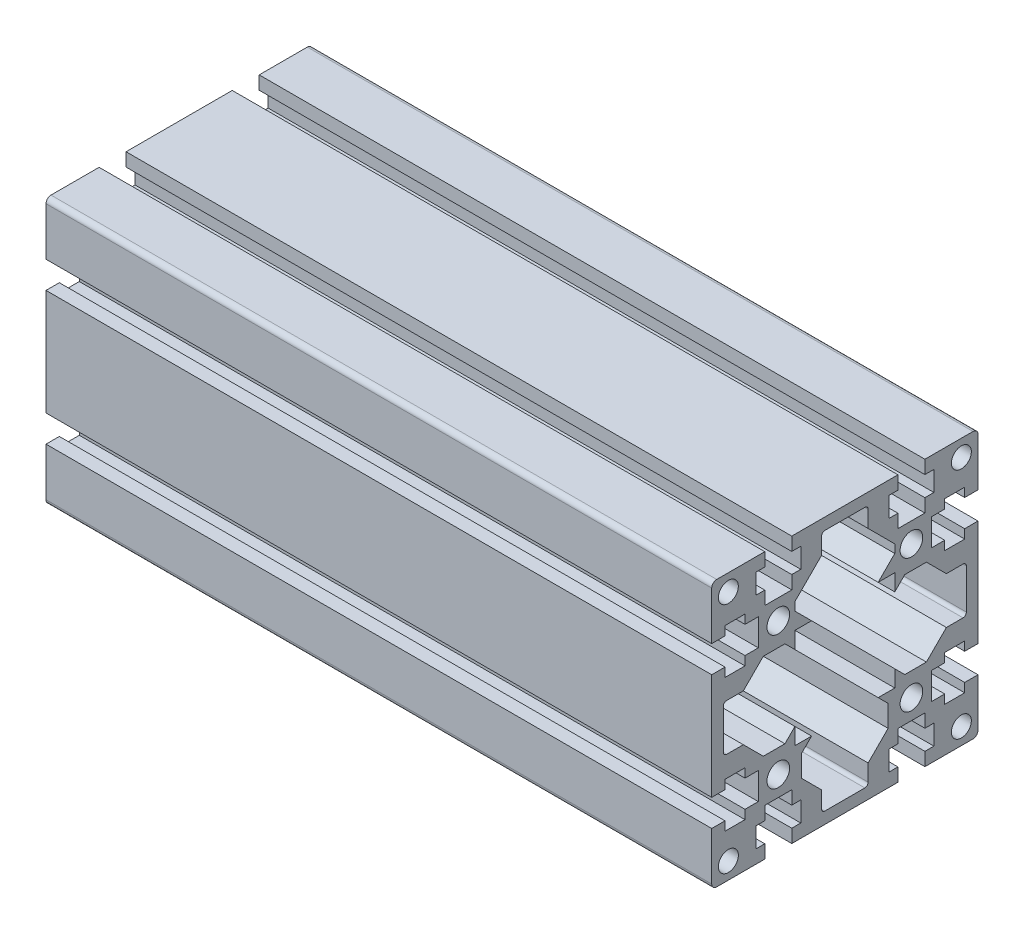
SolidWorks part; units mm, degrees
ref_plane "Front Plane" through (0, 0, 0) normal (0, 0, 1) x (1, 0, 0)
ref_plane "Top Plane" through (0, 0, 0) normal (0, 1, 0) x (1, 0, 0)
ref_plane "Right Plane" through (0, 0, 0) normal (1, 0, 0) x (0, 0, -1)
sketch "草图1" plane through (0, 0, 0) normal (0, 0, 1) x (1, 0, 0)
  line L0 (-530.3448, 0) -> (-330.3448, 0)
  dimension "D1" = 200
other "Aluminium profile 80 X 80G X R1.5(1)"
ref_plane "Plane2" through (-530.3448, 0, 0) normal (1, 0, 0) x (0, 1, 0)
sketch "Sketch1" plane through (-530.3448, 0, 0) normal (1, 0, 0) x (0, 1, 0)
  line L0 (0, 40) -> (0, 0) construction
  line L1 (0, 0) -> (40, 0) construction
  line L2 (-24.05, 40) -> (-24.05, 36)
  line L3 (-38.5, 40) -> (-24.05, 40)
  line L4 (-40, 38.5) -> (-40, 24.05)
  line L5 (-38.5, -40) -> (-24.05, -40)
  line L6 (40, 38.5) -> (40, 24.05)
  line L7 (-24.05, 36) -> (-26.75, 36)
  line L8 (-26.75, 36) -> (-26.75, 30)
  line L9 (-26.75, 30) -> (-24.05, 30)
  line L10 (-24.05, 30) -> (-24.05, 26)
  line L11 (-24.05, 26) -> (-15.95, 26)
  line L12 (-15.95, 26) -> (-15.95, 30)
  line L13 (-15.95, 30) -> (-13.25, 30)
  line L14 (-13.25, 30) -> (-13.25, 36)
  line L15 (-13.25, 36) -> (-15.95, 36)
  line L16 (-15.95, 36) -> (-15.95, 40)
  line L17 (-40, 15.95) -> (-36, 15.95)
  line L18 (-36, 15.95) -> (-36, 13.25)
  line L19 (-15.95, 40) -> (15.95, 40)
  line L20 (-20, 20) -> (-20, 40) construction
  line L21 (20, 20) -> (20, 40) construction
  line L22 (15.95, 36) -> (15.95, 40)
  line L23 (13.25, 36) -> (15.95, 36)
  line L24 (13.25, 30) -> (13.25, 36)
  line L25 (15.95, 30) -> (13.25, 30)
  line L26 (-36, 13.25) -> (-30, 13.25)
  line L27 (-30, 13.25) -> (-30, 15.95)
  line L28 (-26, 15.95) -> (-26, 24.05)
  line L29 (-26, 24.05) -> (-30, 24.05)
  line L30 (-30, 24.05) -> (-30, 26.75)
  line L31 (-30, 26.75) -> (-36, 26.75)
  line L32 (-36, 26.75) -> (-36, 24.05)
  line L33 (-36, 24.05) -> (-40, 24.05)
  line L34 (-30, 15.95) -> (-26, 15.95)
  line L35 (15.95, 26) -> (15.95, 30)
  line L36 (24.05, 26) -> (15.95, 26)
  line L37 (24.05, 30) -> (24.05, 26)
  line L38 (26.75, 30) -> (24.05, 30)
  line L39 (26.75, 36) -> (26.75, 30)
  line L40 (24.05, 36) -> (26.75, 36)
  line L41 (24.05, 40) -> (24.05, 36)
  line L42 (24.05, -40) -> (24.05, -36)
  line L43 (24.05, -36) -> (26.75, -36)
  line L44 (26.75, -36) -> (26.75, -30)
  line L45 (26.75, -30) -> (24.05, -30)
  line L46 (24.05, -30) -> (24.05, -26)
  line L47 (24.05, -26) -> (15.95, -26)
  line L48 (15.95, -26) -> (15.95, -30)
  line L49 (15.95, -30) -> (13.25, -30)
  line L50 (13.25, -30) -> (13.25, -36)
  line L51 (13.25, -36) -> (15.95, -36)
  line L52 (15.95, -36) -> (15.95, -40)
  line L53 (-15.95, -36) -> (-15.95, -40)
  line L54 (-13.25, -36) -> (-15.95, -36)
  line L55 (-13.25, -30) -> (-13.25, -36)
  line L56 (-15.95, -30) -> (-13.25, -30)
  line L57 (-15.95, -26) -> (-15.95, -30)
  line L58 (-24.05, -26) -> (-15.95, -26)
  line L59 (-24.05, -30) -> (-24.05, -26)
  line L60 (-26.75, -30) -> (-24.05, -30)
  line L61 (-26.75, -36) -> (-26.75, -30)
  line L62 (-24.05, -36) -> (-26.75, -36)
  line L63 (-24.05, -40) -> (-24.05, -36)
  line L64 (-30, -15.95) -> (-26, -15.95)
  line L65 (-36, -26.75) -> (-36, -24.05)
  line L66 (-30, -26.75) -> (-36, -26.75)
  line L67 (-30, -24.05) -> (-30, -26.75)
  line L68 (-26, -24.05) -> (-30, -24.05)
  line L69 (-26, -15.95) -> (-26, -24.05)
  line L70 (-30, -13.25) -> (-30, -15.95)
  line L71 (-36, -13.25) -> (-30, -13.25)
  line L72 (-36, -15.95) -> (-36, -13.25)
  line L73 (36, 24.05) -> (40, 24.05)
  line L74 (40, 15.95) -> (36, 15.95)
  line L75 (36, -15.95) -> (36, -13.25)
  line L76 (36, -13.25) -> (30, -13.25)
  line L77 (30, -13.25) -> (30, -15.95)
  line L78 (26, -15.95) -> (26, -24.05)
  line L79 (26, -24.05) -> (30, -24.05)
  line L80 (30, -24.05) -> (30, -26.75)
  line L81 (30, -26.75) -> (36, -26.75)
  line L82 (36, -26.75) -> (36, -24.05)
  line L83 (30, -15.95) -> (26, -15.95)
  line L84 (30, 15.95) -> (26, 15.95)
  line L85 (36, 26.75) -> (36, 24.05)
  line L86 (30, 26.75) -> (36, 26.75)
  line L87 (30, 24.05) -> (30, 26.75)
  line L88 (26, 24.05) -> (30, 24.05)
  line L89 (26, 15.95) -> (26, 24.05)
  line L90 (30, 13.25) -> (30, 15.95)
  line L91 (36, 13.25) -> (30, 13.25)
  line L92 (36, 15.95) -> (36, 13.25)
  line L93 (-36, -15.95) -> (-40, -15.95)
  line L94 (-36, -24.05) -> (-40, -24.05)
  line L95 (36, -15.95) -> (40, -15.95)
  line L96 (36, -24.05) -> (40, -24.05)
  line L97 (-13, 18) -> (-10, 15)
  line L98 (-15, 15) -> (-10, 15)
  line L99 (-15, 15) -> (-15, 10)
  line L100 (-15, -15) -> (-10, -15)
  line L101 (15, 15) -> (15, 10)
  line L102 (-18, 13) -> (-15, 10)
  line L104 (13, 18) -> (10, 15)
  line L105 (13, -18) -> (10, -15)
  line L106 (20, -15) -> (15, -10)
  line L107 (-18, -13) -> (-15, -10)
  line L108 (-13, -18) -> (-10, -15)
  line L109 (15, -10) -> (15, -15)
  line L110 (10, 15) -> (15, 15)
  line L111 (-15, -10) -> (-15, -15)
  line L112 (10, -15) -> (15, -15)
  line L113 (15, 10) -> (20, 15)
  line L235 (24.05, 40) -> (38.5, 40)
  line L249 (-40, 15.95) -> (-40, -15.95)
  line L250 (-20, 20) -> (-26, 20) construction
  line L264 (40, 15.95) -> (40, -15.95)
  line L265 (-13, 24.5) -> (-7, 30.5)
  line L266 (-7, 30.5) -> (-7, 35.5)
  line L267 (7, 35.5) -> (7, 30.5)
  line L268 (7, 30.5) -> (13, 24.5)
  line L269 (-6, -36.5) -> (6, -36.5)
  line L270 (-13, 24.5) -> (-13, 18)
  line L271 (-35.5, 7) -> (-30.5, 7)
  line L272 (-30.5, 7) -> (-24.5, 13)
  line L273 (-24.5, 13) -> (-18, 13)
  line L274 (13, 24.5) -> (13, 18)
  line L275 (-15.95, -40) -> (15.95, -40)
  line L276 (35.5, 7) -> (30.5, 7)
  line L277 (30.5, 7) -> (22.5, 15)
  line L278 (24.05, -40) -> (38.5, -40)
  line L279 (20, 15) -> (22.5, 15)
  line L333 (-13, -24.5) -> (-13, -18)
  line L336 (-13, -24.5) -> (-7, -30.5)
  line L385 (-7, -30.5) -> (-7, -35.5)
  line L386 (-36.5, 6) -> (-36.5, -6)
  line L387 (7, -35.5) -> (7, -30.5)
  line L429 (7, -30.5) -> (13, -24.5)
  line L430 (13, -24.5) -> (13, -18)
  line L494 (20, -15) -> (22.5, -15)
  line L496 (30.5, -7) -> (22.5, -15)
  line L497 (35.5, -7) -> (30.5, -7)
  line L498 (-24.5, -13) -> (-18, -13)
  line L499 (-30.5, -7) -> (-24.5, -13)
  line L500 (-35.5, -7) -> (-30.5, -7)
  line L512 (40, -24.05) -> (40, -38.5)
  line L519 (-40, -24.05) -> (-40, -38.5)
  line L520 (-6, 36.5) -> (6, 36.5)
  line L523 (36.5, 6) -> (36.5, -6)
  circle A0 centre (-20, 20) radius 3.4
  circle A2 centre (20, 20) radius 3.4
  circle A3 centre (20, -20) radius 3.4
  circle A7 centre (-20, -20) radius 3.4
  arc A8 (-38.5, 40) -> (-40, 38.5) centre (-38.5, 38.5) ccw
  arc A9 (-40, -38.5) -> (-38.5, -40) centre (-38.5, -38.5) ccw
  arc A10 (38.5, -40) -> (40, -38.5) centre (38.5, -38.5) ccw
  arc A11 (38.5, 40) -> (40, 38.5) centre (38.5, 38.5) cw
  circle A12 centre (-35, 35) radius 3
  circle A13 centre (35, 35) radius 3
  circle A14 centre (35, -35) radius 3
  arc A15 (-6, 36.5) -> (-7, 35.5) centre (-6, 35.5) ccw
  arc A16 (6, 36.5) -> (7, 35.5) centre (6, 35.5) cw
  arc A17 (-36.5, 6) -> (-35.5, 7) centre (-35.5, 6) cw
  arc A18 (-36.5, -6) -> (-35.5, -7) centre (-35.5, -6) ccw
  arc A19 (36.5, -6) -> (35.5, -7) centre (35.5, -6) cw
  arc A20 (36.5, 6) -> (35.5, 7) centre (35.5, 6) ccw
  arc A21 (6, -36.5) -> (7, -35.5) centre (6, -35.5) ccw
  arc A22 (-6, -36.5) -> (-7, -35.5) centre (-6, -35.5) cw
  point P48 (-20, 20)
  point P97 (0, 0)
  point P104 (-7, 36.5)
  point P185 (40, 40)
  point P187 (40, -40)
  point P188 (-40, -40)
  point P190 (-40, 40)
  dimension "D1" = 80
  dimension "D2" = 80
  dimension "D3" = 20
  dimension "D4" = 8.1
  dimension "D5" = 45
  dimension "D6" = 7
  dimension "D7" = 13.5
  dimension "D8" = 6
  dimension "D12" = 5
  dimension "D13" = 5
  dimension "D14" = 20
  dimension "D18" = 1
  dimension "D19" = 14
  dimension "D15" = 6.8
  dimension "D27" = 45
  dimension "D20" = 1.5
  dimension "D11" = 6
  dimension "D9" = 4
  dimension "D10" = 14
  dimension "D16" = 14
  dimension "D17" = 45
  dimension "D21" = 3.5
  dimension "D22" = 3.5
  dimension "D23" = 73
  dimension "D24" = 30
  dimension "D25" = 30
  dimension "D26" = 45
  dimension "D28" = 5
sketch "Sketch10" plane through (-330.3448, 0, 0) normal (1, 0, 0) x (0, 0, -1)
  circle A0 centre (35, -35) radius 3
  circle A1 centre (-35, -35) radius 3 construction
  circle A2 centre (35, 35) radius 3 construction
  dimension "D1" = 6
  dimension "D2" = 70
  dimension "D3" = 70
extrude "Cut-Extrude1" cut sketch "Sketch10" against normal through all
